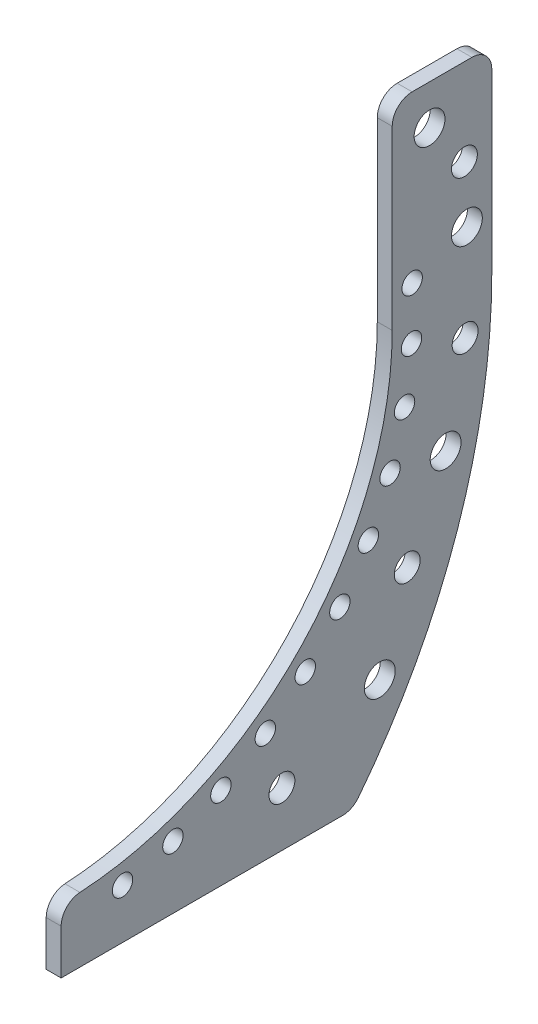
from build123d import *

# Parameters (mm, degrees)
SKETCH_1_R      = 1.55
SKETCH_1_R_2    = 1.025
SKETCH_1_R_3    = 1.3
EXTRUDE_1_DEPTH = 1.5
FILLET_R2_1_R   = 2


with BuildPart() as part:
    # 草图1 → 凸台-拉伸1 (new body)
    with BuildSketch(Plane(origin=(0, 0, 0), x_dir=(0, 0, -1), z_dir=(1, 0, 0))):
        with BuildLine():
            Line((9.25, 19.75), (9.25, 0))
            ThreePointArc((9.25, 0), (-0.488699526, -23.511300474), (-24, -33.25))
            Line((-24, -33.25), (-24, -39.7))
            Line((-24, -39.7), (5.238932767, -39.7))
            ThreePointArc((5.238932767, -39.7), (15.644467461, -21.049940647), (19.25, 0))
            Line((19.25, 0), (19.25, 19.75))
            Line((19.25, 19.75), (9.25, 19.75))
        make_face()
        with Locations((13, 15.75)):
            Circle(SKETCH_1_R, mode=Mode.SUBTRACT)
        with Locations((11.25, 3.116215025)):
            Circle(SKETCH_1_R_2, mode=Mode.SUBTRACT)
        with Locations((-17.835585997, -34.70680769)):
            Circle(SKETCH_1_R_2, mode=Mode.SUBTRACT)
        with Locations((-12.773303956, -33.414424968)):
            Circle(SKETCH_1_R_2, mode=Mode.SUBTRACT)
        with Locations((-7.957653042, -31.387985027)):
            Circle(SKETCH_1_R_2, mode=Mode.SUBTRACT)
        with Locations((-3.494424789, -28.672005254)):
            Circle(SKETCH_1_R_2, mode=Mode.SUBTRACT)
        with Locations((0.518331383, -25.326151034)):
            Circle(SKETCH_1_R_2, mode=Mode.SUBTRACT)
        with Locations((3.992462152, -21.423925006)):
            Circle(SKETCH_1_R_2, mode=Mode.SUBTRACT)
        with Locations((6.851646862, -17.05105234)):
            Circle(SKETCH_1_R_2, mode=Mode.SUBTRACT)
        with Locations((9.033074163, -12.303597496)):
            Circle(SKETCH_1_R_2, mode=Mode.SUBTRACT)
        with Locations((10.488821863, -7.285853861)):
            Circle(SKETCH_1_R_2, mode=Mode.SUBTRACT)
        with Locations((11.1869097, -2.108052596)):
            Circle(SKETCH_1_R_2, mode=Mode.SUBTRACT)
        with Locations((16.57025586, -4.32369512)):
            Circle(SKETCH_1_R_3, mode=Mode.SUBTRACT)
        with Locations((14.615659071, -13.170834237)):
            Circle(SKETCH_1_R, mode=Mode.SUBTRACT)
        with Locations((16.5, 11.05)):
            Circle(SKETCH_1_R_3, mode=Mode.SUBTRACT)
        with Locations((16.75, 5.25)):
            Circle(SKETCH_1_R, mode=Mode.SUBTRACT)
        with Locations((-1.828452918, -34.25)):
            Circle(SKETCH_1_R_3, mode=Mode.SUBTRACT)
        with Locations((8, -29.75)):
            Circle(SKETCH_1_R, mode=Mode.SUBTRACT)
        with Locations((10.756717193, -21.368448937)):
            Circle(SKETCH_1_R_3, mode=Mode.SUBTRACT)
    extrude(amount=EXTRUDE_1_DEPTH)

    # R2 圆角1
    fillet_r2_1_edges = [part.edges().sort_by_distance(p)[0] for p in [
        (0.75, 19.75, -19.25),
        (0.75, -39.7, -5.238932767),
        (0.75, -33.25, 24),
        (0.75, 19.75, -9.25),
    ]]
    fillet(fillet_r2_1_edges, radius=FILLET_R2_1_R)


solid = part.part
